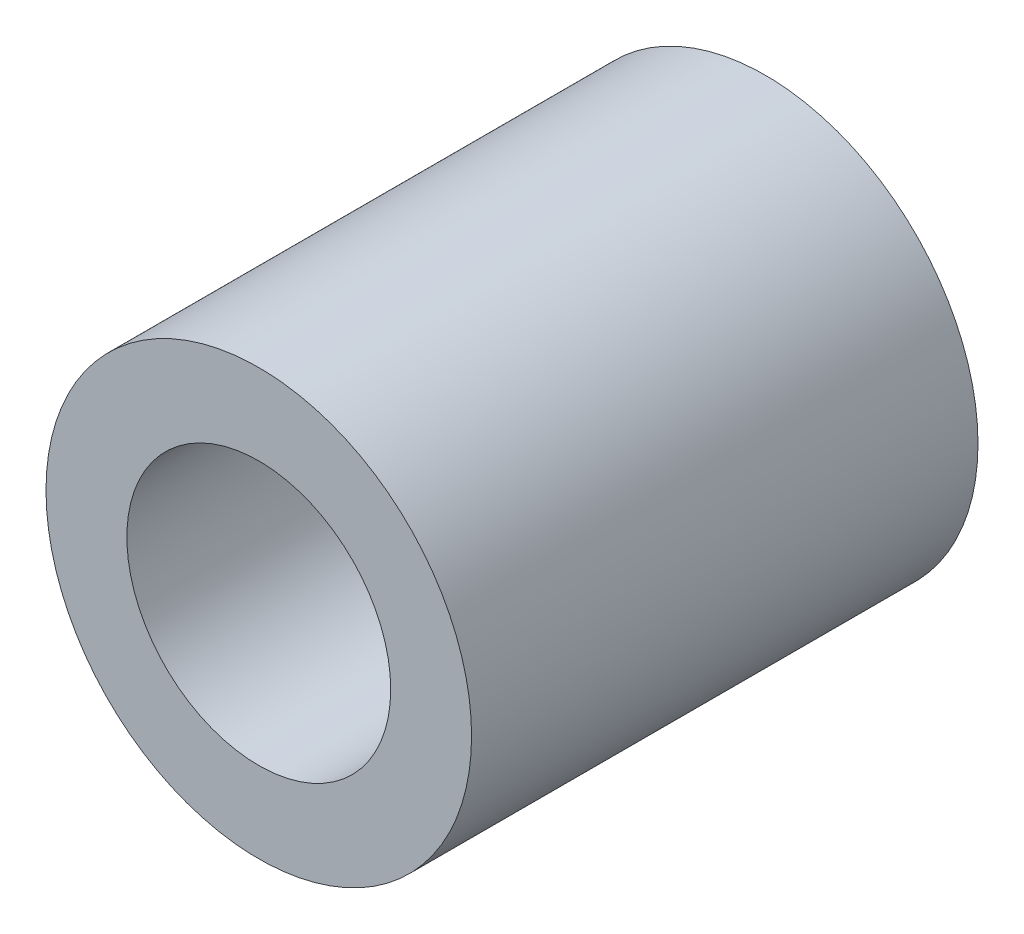
SolidWorks part; units mm, degrees
material "尼龙 101"
ref_plane "前视基准面" through (0, 0, 0) normal (0, 0, 1) x (1, 0, 0)
ref_plane "上视基准面" through (0, 0, 0) normal (0, 1, 0) x (1, 0, 0)
ref_plane "右视基准面" through (0, 0, 0) normal (1, 0, 0) x (0, 0, -1)
other "Configuration Table"
sketch "草图1" plane through (0, 0, 0) normal (0, 0, 1) x (1, 0, 0)
  circle A0 centre (0, 0) radius 1.55
  circle A1 centre (0, 0) radius 2.5
  dimension "D1" = 3.1
  dimension "D2" = 5
extrude "凸台-拉伸1" add sketch "草图1" along normal blind 5.95
